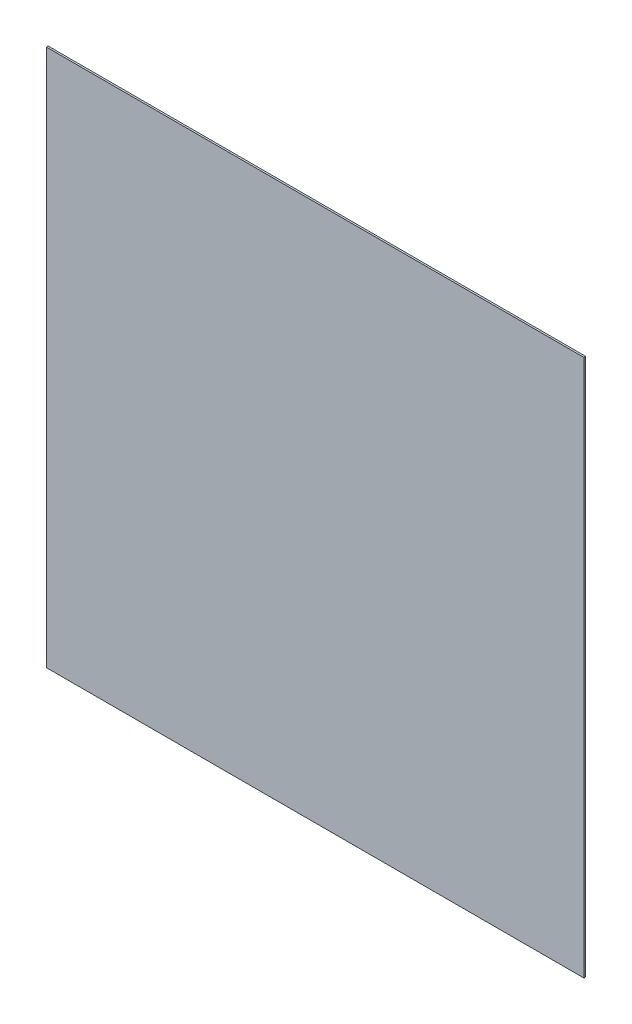
from build123d import *

# Parameters (mm, degrees)
SKETCH_1_W      = 600
SKETCH_1_H      = 600
EXTRUDE_1_DEPTH = 2


with BuildPart() as part:
    # 草图1 → 凸台-拉伸1 (new body)
    with BuildSketch(Plane.XY):
        Rectangle(SKETCH_1_W, SKETCH_1_H)
    extrude(amount=EXTRUDE_1_DEPTH)


solid = part.part
